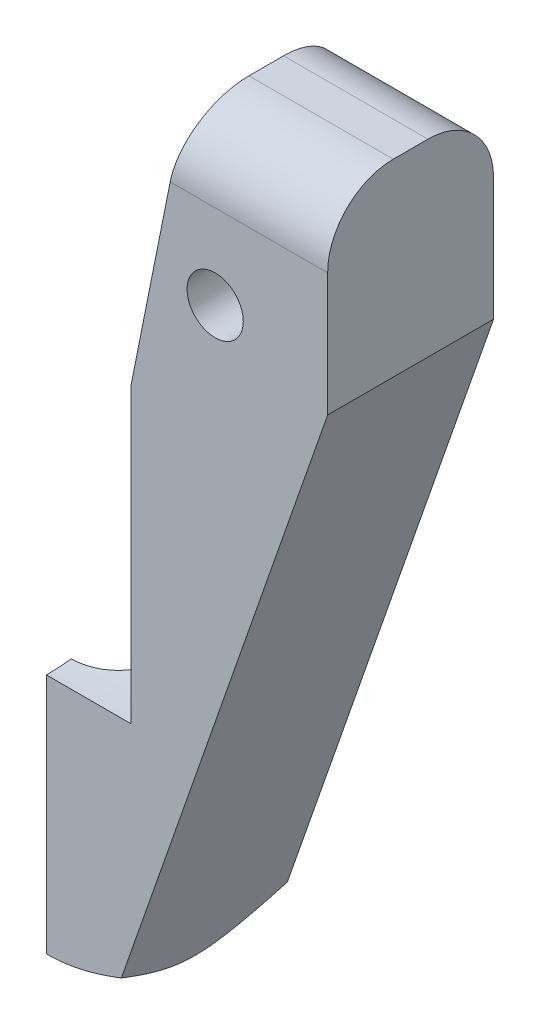
SolidWorks part; units mm, degrees
ref_plane "Front Plane" through (0, 0, 0) normal (0, 0, 1) x (1, 0, 0)
ref_plane "Top Plane" through (0, 0, 0) normal (0, 1, 0) x (1, 0, 0)
ref_plane "Right Plane" through (0, 0, 0) normal (1, 0, 0) x (0, 0, -1)
sketch "Sketch1" plane through (0, 0, 0) normal (0, 0, 1) x (1, 0, 0)
  line L22 (39, -51.5036) -> (34.8377, -51.5036)
  line L23 (39, -28) -> (39, -51.5036)
  line L24 (44.6, 0) -> (39, -28)
  line L25 (60, -20.1364) -> (60, 0)
  line L26 (60, -20.1364) -> (38.9512, -80.4124)
  line L27 (60, 0) -> (44.6, 0)
  line L28 (21.0488, -80.4124) -> (0, -20.1364)
  line L29 (0, -20.1364) -> (0, 0)
  line L30 (21, -51.5036) -> (21, -28.6)
  line L31 (25.1623, -51.5036) -> (21, -51.5036)
  line L32 (21, -28.6) -> (15.3764, 0)
  line L33 (0, 0) -> (15.3764, 0)
  line L34 (37, -86) -> (23, -86)
  line L35 (25.1623, -51.5036) -> (34.8377, -51.5036)
  circle A0 centre (48, -16) radius 3
  circle A1 centre (12, -16) radius 3
  spline S0 degree 3 poles (38.9512, -80.4124) (38.741, -81.0144) (38.5334, -81.6089) (38.3309, -82.1888) knots 0 0 0 0 0.25 0.25 0.25 0.25
  spline S1 degree 3 poles (38.3309, -82.1888) (38.1284, -82.7688) (37.9302, -83.3362) (37.7441, -83.869) knots 0.25 0.25 0.25 0.25 0.5 0.5 0.5 0.5
  spline S2 degree 3 poles (37.7441, -83.869) (37.6511, -84.1355) (37.5613, -84.3926) (37.4767, -84.6348) knots 0.5 0.5 0.5 0.5 0.625 0.625 0.625 0.625
  spline S3 degree 3 poles (37.4767, -84.6348) (37.3922, -84.877) (37.3127, -85.1045) (37.2423, -85.3061) knots 0.625 0.625 0.625 0.625 0.75 0.75 0.75 0.75
  spline S4 degree 3 poles (37.2423, -85.3061) (37.1719, -85.5076) (37.1112, -85.6816) (37.0682, -85.8048) knots 0.75 0.75 0.75 0.75 0.875 0.875 0.875 0.875
  spline S5 degree 2 poles (37.0682, -85.8048) (37.0252, -85.9279) (37, -86) knots 0.875 0.875 0.875 1 1 1
  spline S6 degree 2 poles (23, -86) (22.9755, -85.9299) (22.9325, -85.8066) knots 0 0 0 0.125 0.125 0.125
  spline S7 degree 3 poles (22.9325, -85.8066) (22.911, -85.745) (22.8847, -85.6697) (22.8553, -85.5855) knots 0.125 0.125 0.125 0.125 0.1875 0.1875 0.1875 0.1875
  spline S8 degree 3 poles (22.8553, -85.5855) (22.8258, -85.5013) (22.7932, -85.4079) (22.7583, -85.3078) knots 0.1875 0.1875 0.1875 0.1875 0.25 0.25 0.25 0.25
  spline S9 degree 3 poles (22.7583, -85.3078) (22.6883, -85.1074) (22.6089, -84.8801) (22.524, -84.637) knots 0.25 0.25 0.25 0.25 0.375 0.375 0.375 0.375
  spline S10 degree 3 poles (22.524, -84.637) (22.4392, -84.3939) (22.3487, -84.1348) (22.2555, -83.8681) knots 0.375 0.375 0.375 0.375 0.5 0.5 0.5 0.5
  spline S11 degree 3 poles (22.2555, -83.8681) (22.0692, -83.3346) (21.8716, -82.7687) (21.6691, -82.1889) knots 0.5 0.5 0.5 0.5 0.75 0.75 0.75 0.75
  spline S12 degree 3 poles (21.6691, -82.1889) (21.4667, -81.6091) (21.2591, -81.0146) (21.0488, -80.4124) knots 0.75 0.75 0.75 0.75 1 1 1 1
  dimension "D1" = 36
  dimension "D2" = 16
  dimension "D3" = 12
  dimension "D4" = 12
extrude "Boss-Extrude2" add sketch "Sketch1" along normal blind 17.7
ref_plane "Plane2" through (30, 0, 0) normal (-1, 0, 0) x (0, 0, 1)
sketch "Sketch2" plane through (30, 0, 0) normal (-1, 0, 0) x (0, 0, 1)
  line L0 (11.5, -86) -> (11.5, -81.75)
  line L1 (17.7, -86) -> (0, -86) construction
  line L2 (15.0441, -75) -> (15.0441, -57.48)
  line L3 (102, 6.2) -> (84.4804, 6.2)
  line L4 (113, 2.65) -> (108.7541, 2.65)
  line L5 (11.5, -86) -> (8.85, -86)
  line L6 (8.85, -86) -> (8.85, -57.48)
  line L7 (8.85, -57.48) -> (15.0441, -57.48)
  arc A0 (107.1067, 3.5159) -> (108.7541, 2.65) centre (108.7541, 4.65) ccw
  arc A1 (107.1067, 3.5159) -> (102, 6.2) centre (102, 0) ccw
  arc A2 (11.5, -81.75) -> (12.3644, -80.1037) centre (13.5, -81.75) cw
  arc A3 (12.3644, -80.1037) -> (15.0441, -75) centre (8.8441, -75) ccw
  point P8 (8.85, -86)
  dimension "D1" = 4.25
  dimension "D2" = 2
  dimension "D3" = 6.2
  dimension "D4" = 28.52
  dimension "D5" = 17.52
  dimension "D6" = 2.65
revolve "Cut-Revolve2" cut sketch "Sketch2" angle 360 about L6
sketch "Sketch3" plane through (30, 0, 0) normal (-1, 0, 0) x (0, 0, 1)
  line L0 (17.7, -20.1364) -> (17.7, -80.4124) construction
  line L2 (0, -51.5036) -> (17.7, -51.5036)
  line L3 (17.7, -51.5036) -> (17.7, -59.1523)
  line L4 (2.6559, -57.48) -> (15.0441, -57.48) construction
  spline S0 degree 2 poles (17.7, -59.1523) (7.3354, -59.0089) (0, -51.5036) knots 0 0 0 1 1 1
extrude "Cut-Extrude1" cut sketch "Sketch3" against normal up to surface and the other way up to surface up to face at (39, -39.7518, 8.85) other way up to face at (21, -40.0518, 8.85)
sketch "Sketch4" plane through (30, 0, 0) normal (-1, 0, 0) x (0, 0, 1)
  line L0 (4.1824, -56.4823) -> (-7.4784, -54.9866)
ref_plane "Plane4" through (0, 0, 8.85) normal (0, 0, -1) x (-1, 0, 0)
sketch "Sketch6" plane through (0, 0, 8.85) normal (0, 0, -1) x (-1, 0, 0)
  line L1 (-30, -56.4823) -> (-30, -54.9866) construction
  ellipse E0 centre (-30, -47.9683) end of major axis (-30, -35.7103) minor radius 6.4919
extrude "Cut-Extrude2" cut sketch "Sketch6" along normal blind 48.7
sketch "Sketch7" plane through (0, 0, 0) normal (0, 1, 0) x (1, 0, 0)
  circle A0 centre (30, -8.85) radius 6.1941
extrude "Cut-Extrude3" cut sketch "Sketch7" against normal blind 60.7
ref_plane "Plane5" through (6, 0, 0) normal (-1, 0, 0) x (0, 0, 1)
sketch "Sketch8" plane through (6, 0, 0) normal (-1, 0, 0) x (0, 0, 1)
  line L0 (17.7, 0) -> (0, 0) construction
  line L1 (17.7, -86) -> (0, -86) construction
  circle A0 centre (8.85, -5) radius 4
  point P7 (8.85, -86)
  dimension "D1" = 8
  dimension "D2" = 5
extrude "Cut-Extrude4" cut sketch "Sketch8" against normal blind 48
fillet "Fillet1" radius 7 4 edges at (52.3, 0, 17.7) (52.3, 0, 0) (7.6882, 0, 0) (7.6882, 0, 17.7)
sketch "Sketch10" plane through (0, -86, 0) normal (0, -1, 0) x (1, 0, 0)
  circle A0 centre (30, 8.85) radius 7
  dimension "D1" = 14
extrude "Cut-Extrude5" cut sketch "Sketch10" against normal blind 48 draft 60 flip side to cut
ref_plane "Plane6" through (0, -5, 0) normal (0, 1, 0) x (1, 0, 0)
sketch "Sketch12" plane through (0, 0, 17.7) normal (0, 0, 1) x (1, 0, 0)
  line L0 (30, -86) -> (30, 13.7307)
  line L1 (23, -86) -> (37, -86) construction
  line L5 (30, -86) -> (-8.2821, -99.4777)
  line L6 (-8.2821, -99.4777) -> (-24.442, 10.8614)
  line L7 (-24.442, 10.8614) -> (30, 13.7307)
extrude "Cut-Extrude8" cut sketch "Sketch12" against normal blind 44 contours L6 L7 L0 L5
